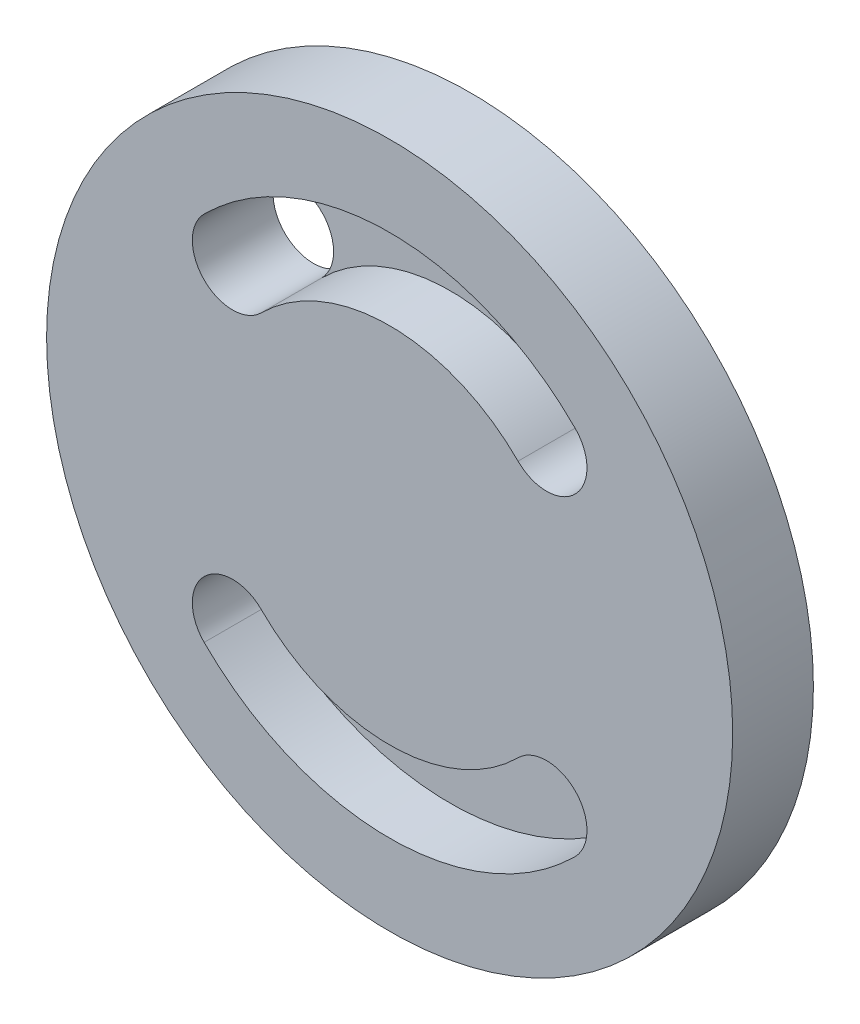
SolidWorks part; units mm, degrees
ref_plane "Front Plane" through (0, 0, 0) normal (0, 0, 1) x (1, 0, 0)
ref_plane "Top Plane" through (0, 0, 0) normal (0, 1, 0) x (1, 0, 0)
ref_plane "Right Plane" through (0, 0, 0) normal (1, 0, 0) x (0, 0, -1)
other "Configuration Table"
sketch "Sketch1" plane through (0, 0, 0) normal (0, 0, 1) x (1, 0, 0)
  circle A0 centre (0, 0) radius 17
  dimension "D1" = 34
extrude "Boss-Extrude1" add sketch "Sketch1" along normal blind 4
sketch "Sketch2" plane through (0, 0, 4) normal (0, 0, 1) x (1, 0, 0)
  line L0 (0, 0) -> (0, 11) construction
  line L1 (0, 0) -> (-7.7782, 7.7782) construction
  circle A0 centre (0, 0) radius 11 construction
  arc A1 (-7.7782, 7.7782) -> (7.7782, 7.7782) centre (0, 0) cw construction
  arc A2 (9.1924, 9.1924) -> (-9.1924, 9.1924) centre (0, 0) ccw
  arc A3 (6.364, 6.364) -> (-6.364, 6.364) centre (0, 0) ccw
  arc A4 (6.364, 6.364) -> (9.1924, 9.1924) centre (7.7782, 7.7782) ccw
  arc A5 (-9.1924, 9.1924) -> (-6.364, 6.364) centre (-7.7782, 7.7782) ccw
  point P6 (0, 11)
  dimension "D1" = 22
  dimension "D2" = 13
  dimension "D3" = 45
extrude "Cut-Extrude1" cut sketch "Sketch2" against normal blind 3
sketch "Sketch3" plane through (0, 0, 4) normal (0, 0, 1) x (1, 0, 0)
  circle A0 centre (7.7782, 7.7782) radius 2
  circle A1 centre (-7.7782, 7.7782) radius 2
  arc A2 (-9.1924, 9.1924) -> (-6.364, 6.364) centre (-7.7782, 7.7782) ccw construction
extrude "Cut-Extrude2" cut sketch "Sketch3" against normal blind 4
sketch "Sketch4" plane through (0, 0, 4) normal (0, 0, 1) x (1, 0, 0)
  line L0 (0, 0) -> (0, -11) construction
  line L1 (7.7782, -7.7782) -> (0, 0) construction
  circle A0 centre (0, 0) radius 11 construction
  arc A1 (-7.7782, -7.7782) -> (7.7782, -7.7782) centre (0, 0) ccw construction
  arc A2 (-9.1924, -9.1924) -> (9.1924, -9.1924) centre (0, 0) ccw
  arc A3 (-6.364, -6.364) -> (6.364, -6.364) centre (0, 0) ccw
  arc A4 (-6.364, -6.364) -> (-9.1924, -9.1924) centre (-7.7782, -7.7782) ccw
  arc A5 (9.1924, -9.1924) -> (6.364, -6.364) centre (7.7782, -7.7782) ccw
  point P6 (0, -11)
  dimension "D1" = 22
  dimension "D3" = 2
  dimension "D2" = 45
extrude "Cut-Extrude3" cut sketch "Sketch4" against normal blind 3
sketch "Sketch7" plane through (0, 0, 0) normal (0, 0, -1) x (-1, 0, 0)
  line L0 (0, 0) -> (0, 5.1005) construction
  circle A0 centre (11, 0) radius 1.5
  circle A1 centre (-11, 0) radius 1.5
  dimension "D1" = 3
  dimension "D2" = 11
extrude "Boss-Extrude3" add sketch "Sketch7" along normal blind 2
